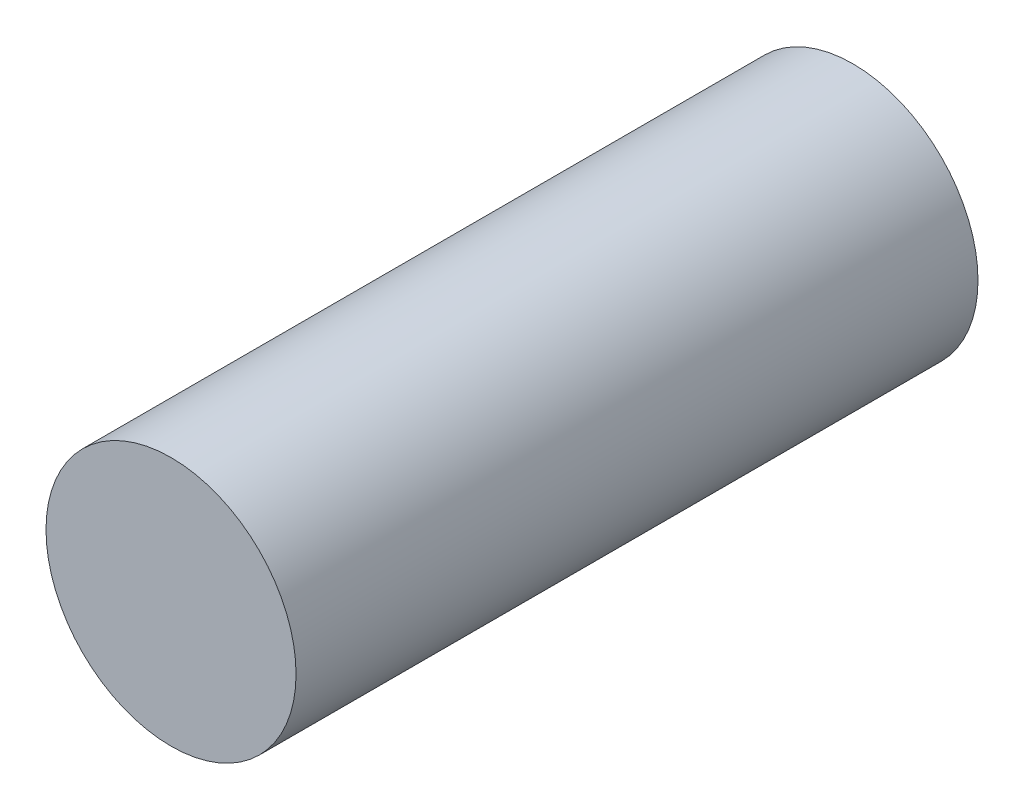
from build123d import *

# Parameters (mm, degrees)
SKETCH1_R           = 0.55
BOSS_EXTRUDE1_DEPTH = 1.5


with BuildPart() as part:
    # Sketch1 → Boss-Extrude1 (new, symmetric)
    with BuildSketch(Plane.XY):
        Circle(SKETCH1_R)
    extrude(amount=BOSS_EXTRUDE1_DEPTH, both=True)


solid = part.part
